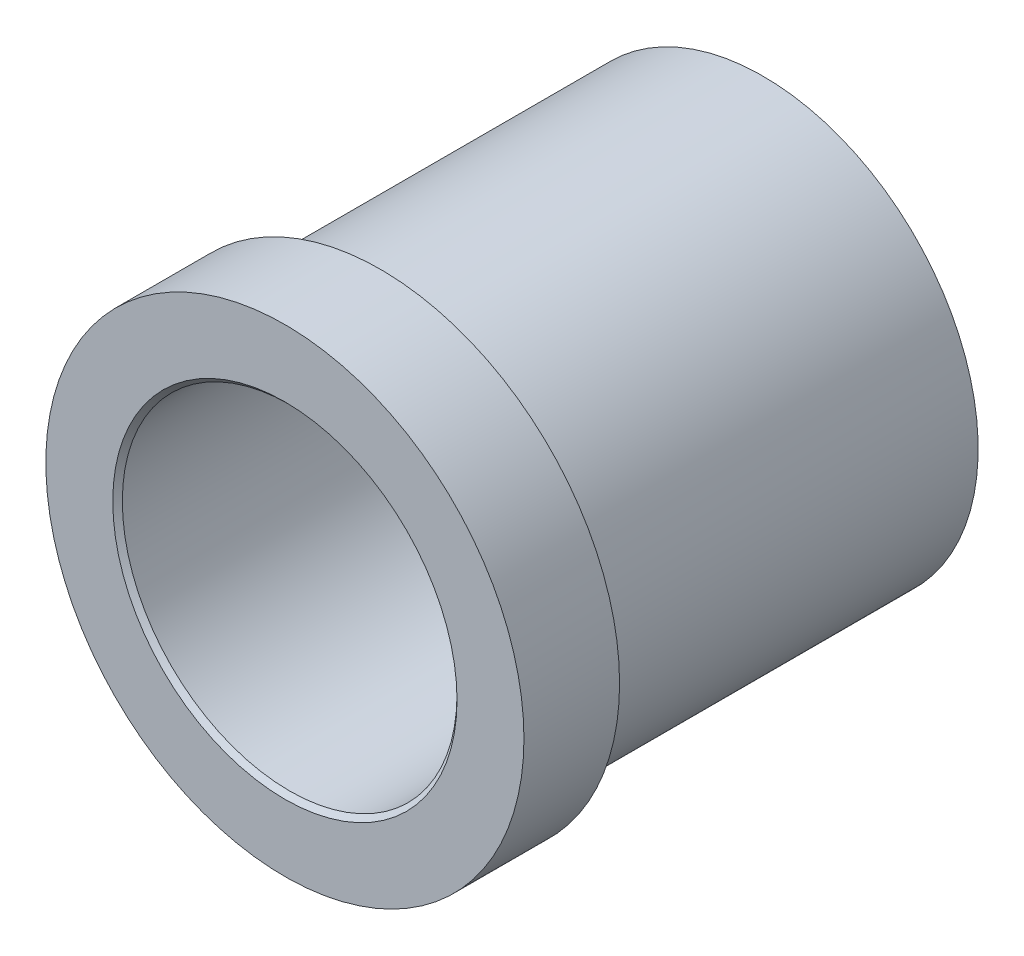
SolidWorks part; units mm, degrees
material "1023 碳钢板 (SS)"
ref_plane "前视基准面" through (0, 0, 0) normal (0, 0, 1) x (1, 0, 0)
ref_plane "上视基准面" through (0, 0, 0) normal (0, 1, 0) x (1, 0, 0)
ref_plane "右视基准面" through (0, 0, 0) normal (1, 0, 0) x (0, 0, -1)
sketch "草图1" plane through (0, 0, 0) normal (0, 0, 1) x (1, 0, 0)
  circle A0 centre (0, 0) radius 25
  dimension "D1" = 50
extrude "凸台-拉伸1" add sketch "草图1" along normal blind 10
sketch "草图2" plane through (0, 0, 0) normal (0, 0, -1) x (-1, 0, 0)
  circle A0 centre (0, 0) radius 22.5
  dimension "D1" = 45
extrude "凸台-拉伸2" add sketch "草图2" along normal blind 40
sketch "草图3" plane through (0, 0, -40) normal (0, 0, -1) x (-1, 0, 0)
  circle A0 centre (0, 0) radius 17.5
  dimension "D1" = 35
extrude "切除-拉伸1" cut sketch "草图3" against normal blind 80
chamfer "倒角1" distance 0.5 angle 45 1 edges at (17.5, 0, 10)
